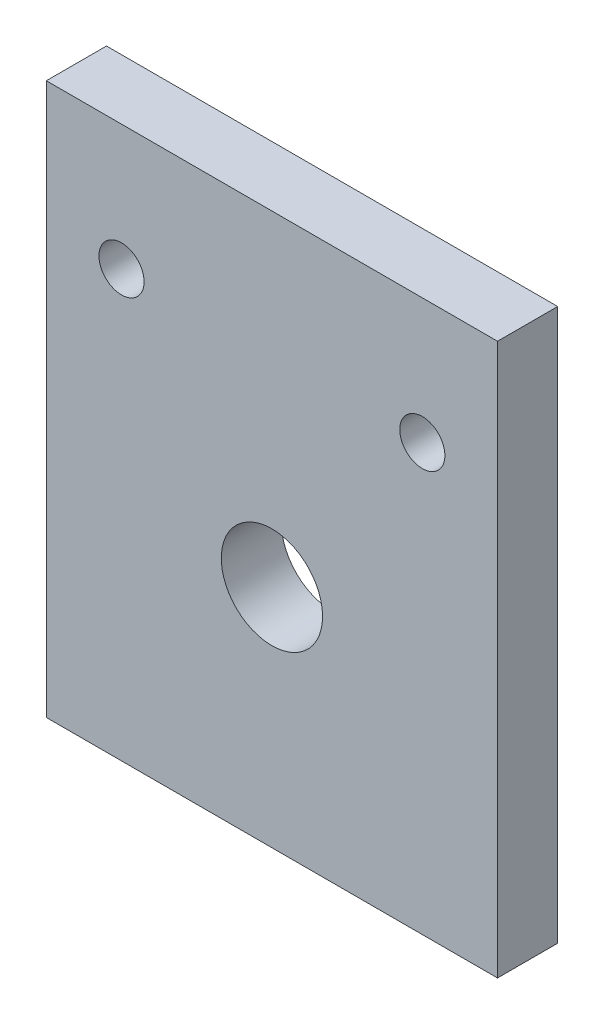
SolidWorks part; units mm, degrees
ref_plane "前视基准面" through (0, 0, 0) normal (0, 0, 1) x (1, 0, 0)
ref_plane "上视基准面" through (0, 0, 0) normal (0, 1, 0) x (1, 0, 0)
ref_plane "右视基准面" through (0, 0, 0) normal (1, 0, 0) x (0, 0, -1)
other "Configuration Table"
sketch "草图1" plane through (0, 0, 0) normal (0, 0, 1) x (1, 0, 0)
  line L0 (-45, -55) -> (45, -55)
  line L1 (45, -55) -> (45, 55)
  line L2 (45, 55) -> (-45, 55)
  line L3 (-45, 55) -> (-45, -55)
  point P0 (0, 0)
  dimension "D1" = 45
  dimension "D2" = 90
  dimension "D3" = 55
  dimension "D4" = 110
extrude "凸台-拉伸1" add sketch "草图1" against normal mid plane 12
sketch "草图2" plane through (0, 0, 0) normal (0, 0, 1) x (1, 0, 0)
  circle A0 centre (-30, 30) radius 4.5
  circle A1 centre (30, 30) radius 4.5
  circle A2 centre (0, -10) radius 10.1
  point P0 (0, 0)
  dimension "D1" = 20.2
  dimension "D2" = 9
  dimension "D3" = 9
  dimension "D4" = 30
  dimension "D5" = 60
  dimension "D6" = 10
  dimension "D7" = 40
extrude "切除-拉伸1" cut sketch "草图2" against normal mid plane 32
